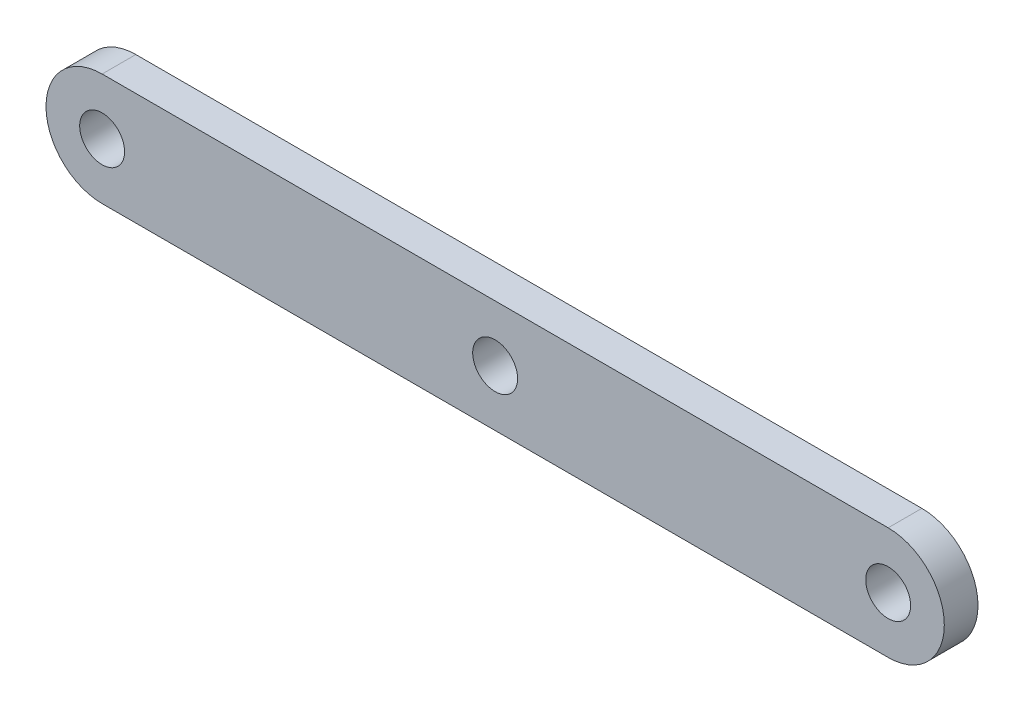
SolidWorks part; units mm, degrees
ref_plane "Front Plane" through (0, 0, 0) normal (0, 0, 1) x (1, 0, 0)
ref_plane "Top Plane" through (0, 0, 0) normal (0, 1, 0) x (1, 0, 0)
ref_plane "Right Plane" through (0, 0, 0) normal (1, 0, 0) x (0, 0, -1)
sketch "Sketch1" plane through (0, 0, 0) normal (0, 0, 1) x (1, 0, 0)
  line L0 (55, 0) -> (-55, 0) construction
  line L1 (0, 10) -> (140, 10)
  line L2 (0, 0) -> (158.2009, 0) construction
  line L3 (0, -10) -> (140, -10)
  arc A0 (0, 10) -> (0, -10) centre (0, 0) ccw
  arc A1 (140, -10) -> (140, 10) centre (140, 0) ccw
  dimension "D1" = 140
  dimension "D2" = 20
  dimension "D3" = 20
extrude "Boss-Extrude1" add sketch "Sketch1" along normal blind 6
sketch "Sketch2" plane through (0, 0, 6) normal (0, 0, 1) x (1, 0, 0)
  circle A0 centre (0, 0) radius 4
  circle A1 centre (140, 0) radius 4
  dimension "D1" = 8
  dimension "D2" = 8
extrude "Cut-Extrude1" cut sketch "Sketch2" against normal blind 95
sketch "Sketch3" plane through (0, 0, 6) normal (0, 0, 1) x (1, 0, 0)
  line L0 (0, 0) -> (140, 0) construction
  circle A0 centre (70, 0) radius 4
  dimension "8" = 8
extrude "Cut-Extrude2" cut sketch "Sketch3" against normal blind 10
